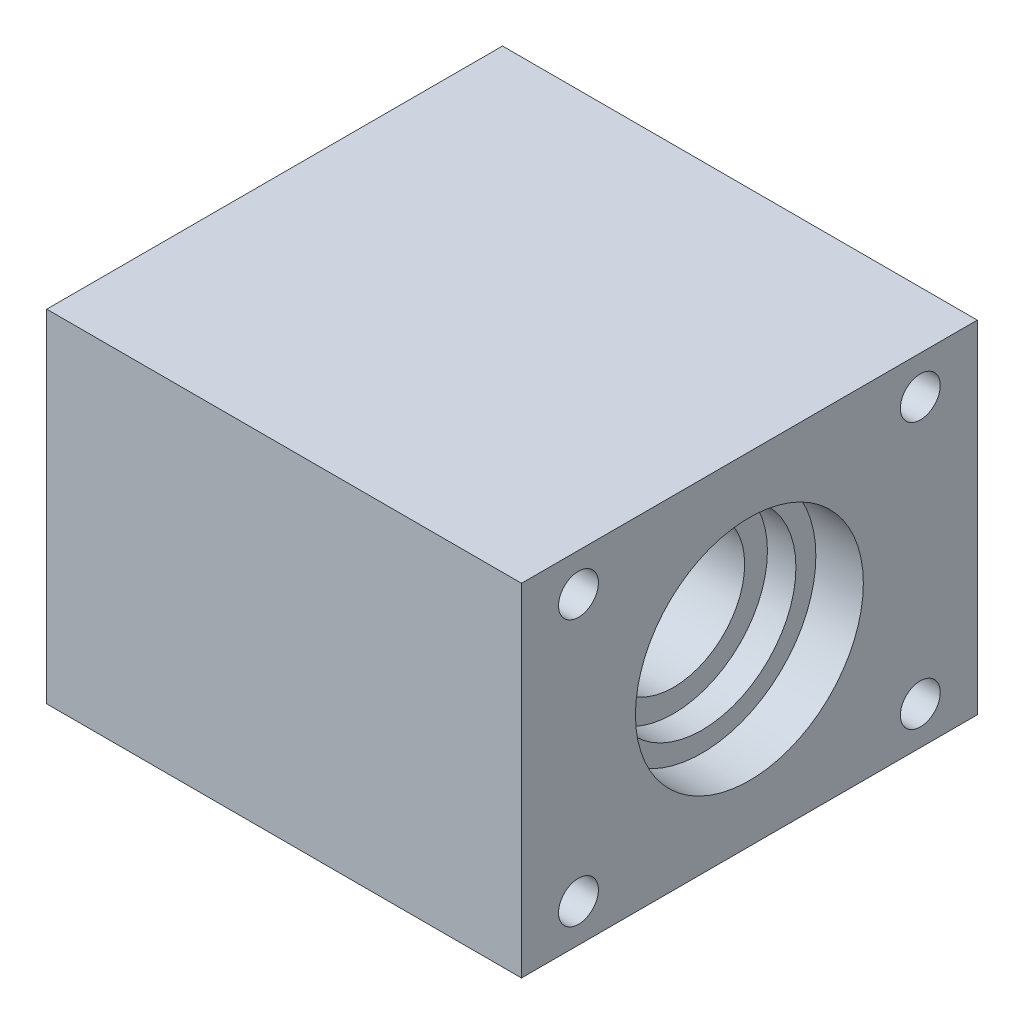
SolidWorks part; units mm, degrees
ref_plane "Front Plane" through (0, 0, 0) normal (0, 0, 1) x (1, 0, 0)
ref_plane "Top Plane" through (0, 0, 0) normal (0, 1, 0) x (1, 0, 0)
ref_plane "Right Plane" through (0, 0, 0) normal (1, 0, 0) x (0, 0, -1)
sketch "Sketch1" plane through (0, 0, 0) normal (1, 0, 0) x (0, 0, -1)
  line L1 (-24, -18) -> (24, -18)
  line L2 (-24, -18) -> (-24, 18)
  line L3 (-24, 18) -> (24, 18)
  line L4 (24, -18) -> (24, 18)
  line L5 (-24, -18) -> (24, 18) construction
  line L6 (-24, 18) -> (24, -18) construction
  circle A1 centre (0, 0) radius 7.5
  dimension "D1" = 48
  dimension "D2" = 15
  dimension "D3" = 36
extrude "Boss-Extrude1" add sketch "Sketch1" along normal mid plane 50
sketch "Sketch2" plane through (-25, 0, 0) normal (-1, 0, 0) x (0, 0, 1)
  circle A0 centre (0, 0) radius 12
  dimension "D1" = 24
extrude "Cut-Extrude1" cut sketch "Sketch2" against normal blind 5
sketch "Sketch3" plane through (-20, 0, 0) normal (-1, 0, 0) x (0, 0, 1)
  circle A0 centre (0, 0) radius 9.9
  dimension "D1" = 19.8
extrude "Cut-Extrude2" cut sketch "Sketch3" against normal blind 3
mirror "Mirror4" about plane through (0, 0, 0) normal (1, 0, 0) of "Cut-Extrude2", "Cut-Extrude1"
sketch "Sketch5" plane through (0, 0, -24) normal (0, 0, -1) x (-1, 0, 0)
  line L1 (0, 0) -> (0, 13.862) construction
  circle A0 centre (7, 0) radius 2
  circle A1 centre (-7, 0) radius 2
  dimension "D2" = 4
  dimension "D1" = 14
extrude "Cut-Extrude3" cut sketch "Sketch5" against normal blind 20
hole_wizard "M5 Tapped Hole1" positions "Sketch6" profile "Sketch7" tap size "M5" standard "ISO"
sketch "Sketch6" plane through (25, 0, 0) normal (1, 0, 0) x (0, 0, -1)
  line L0 (0, 0) -> (0, 29.7992) construction
  line L2 (0, 0) -> (36.2586, 0) construction
  point P0 (-18, 14)
  point P2 (18, 14)
  point P4 (-18, -14)
  point P6 (18, -14)
  dimension "D1" = 28
  dimension "D2" = 36
sketch "Sketch7" plane through (25, 14, 18) normal (0, 1, 0) x (0, 0, -1)
  line L0 (0, 0) -> (0, 13.6618)
  line L1 (0, 13.6618) -> (2.1, 12.4)
  line L2 (2.1, 12.4) -> (2.1, 0)
  line L5 (2.1, 0) -> (0, 0)
  line L10 (0, 13.6618) -> (-2.1, 12.4) construction
  line L11 (0, -6.35) -> (0, 107.95) construction
  dimension "螺纹孔钻头直径" = 4.2
  dimension "螺纹孔钻头深度" = 12.4
  dimension "导头角度" = 118
cosmetic thread "Cosmetic Thread1" parameters "D1"=10, "D2"=5
cosmetic thread "Cosmetic Thread2" parameters "D1"=10, "D2"=5
cosmetic thread "Cosmetic Thread3" parameters "D1"=10, "D2"=5
cosmetic thread "Cosmetic Thread4" parameters "D1"=10, "D2"=5
sketch "Sketch8" plane through (-25, 0, 0) normal (-1, 0, 0) x (0, 0, 1)
hole_wizard "M3 Tapped Hole1" positions "Sketch10" profile "Sketch11" tap size "M3" standard "ISO"
sketch "Sketch10" plane through (-25, 0, 0) normal (-1, 0, 0) x (0, 0, 1)
  line L0 (0, 0) -> (0, 25.5791) construction
  line L2 (0, 0) -> (34.9667, 0) construction
  point P0 (-14, 14)
  point P2 (-14, -14)
  point P4 (14, 14)
  point P6 (14, -14)
  dimension "D1" = 28
  dimension "D2" = 28
sketch "Sketch11" plane through (-25, 14, -14) normal (0, 1, 0) x (0, 0, 1)
  line L0 (0, 0) -> (0, 10.8511)
  line L1 (0, 10.8511) -> (1.25, 10.1)
  line L2 (1.25, 10.1) -> (1.25, 0)
  line L5 (1.25, 0) -> (0, 0)
  line L10 (0, 10.8511) -> (-1.25, 10.1) construction
  line L11 (0, -6.35) -> (0, 107.95) construction
  dimension "螺纹孔钻头直径" = 2.5
  dimension "螺纹孔钻头深度" = 10.1
  dimension "导头角度" = 118
cosmetic thread "Cosmetic Thread5" parameters "D1"=6, "D2"=3
cosmetic thread "Cosmetic Thread6" parameters "D1"=6, "D2"=3
cosmetic thread "Cosmetic Thread7" parameters "D1"=6, "D2"=3
cosmetic thread "Cosmetic Thread8" parameters "D1"=6, "D2"=3
